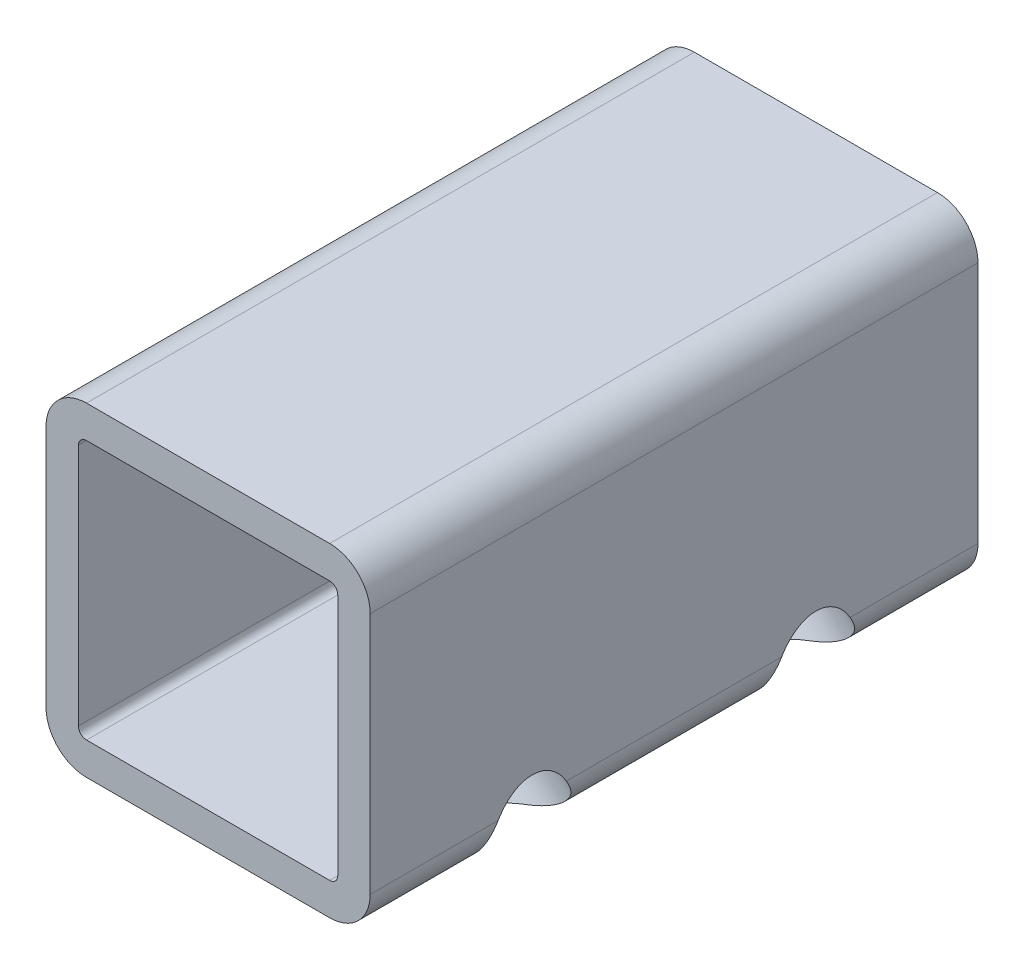
SolidWorks part; units mm, degrees
material "1023 碳钢板 (SS)"
ref_plane "Front Plane" through (0, 0, 0) normal (0, 0, 1) x (1, 0, 0)
ref_plane "Top Plane" through (0, 0, 0) normal (0, 1, 0) x (1, 0, 0)
ref_plane "Right Plane" through (0, 0, 0) normal (1, 0, 0) x (0, 0, -1)
sketch "Sketch1" plane through (0, 0, 0) normal (0, 0, 1) x (1, 0, 0)
  line L0 (-15, 16) -> (15, 16)
  line L1 (-15, 20) -> (15, 20)
  line L2 (-20, 15) -> (-20, -15)
  line L3 (-15, -20) -> (15, -20)
  line L4 (20, 15) -> (20, -15)
  line L5 (-20, 20) -> (20, -20) construction
  line L6 (-20, -20) -> (20, 20) construction
  line L7 (16, 15) -> (16, -15)
  line L8 (-15, -16) -> (15, -16)
  line L9 (-16, 15) -> (-16, -15)
  arc A0 (-20, -15) -> (-15, -20) centre (-15, -15) ccw
  arc A1 (15, -20) -> (20, -15) centre (15, -15) ccw
  arc A2 (15, 20) -> (20, 15) centre (15, 15) cw
  arc A3 (-15, 20) -> (-20, 15) centre (-15, 15) ccw
  arc A4 (15, 16) -> (16, 15) centre (15, 15) cw
  arc A5 (15, -16) -> (16, -15) centre (15, -15) ccw
  arc A6 (-16, -15) -> (-15, -16) centre (-15, -15) ccw
  arc A7 (-15, 16) -> (-16, 15) centre (-15, 15) ccw
  point P0 (0, 0)
  dimension "D3" = 5
  dimension "D1" = 40
  dimension "D2" = 40
  dimension "D4" = 4
extrude "Boss-Extrude1" add sketch "Sketch1" along normal blind 75 contours L0 A7 L9 A6 L8 A5 L7 A4 | L2 A0 L3 A1 L4 A2 L1 A3
ref_plane "Plane1" through (0, 0, 0) normal (-0.7071, 0.7071, 0) x (0, 0, 1)
sketch "Sketch2" plane through (0, 0, 0) normal (-0.7071, 0.7071, 0) x (0, 0, 1)
  circle A0 centre (20, 0) radius 5.5
  circle A1 centre (55, 0) radius 5.5
  dimension "D1" = 11
  dimension "D2" = 11
  dimension "D3" = 20
  dimension "D4" = 35
extrude "Cut-Extrude1" cut sketch "Sketch2" against normal blind 45
